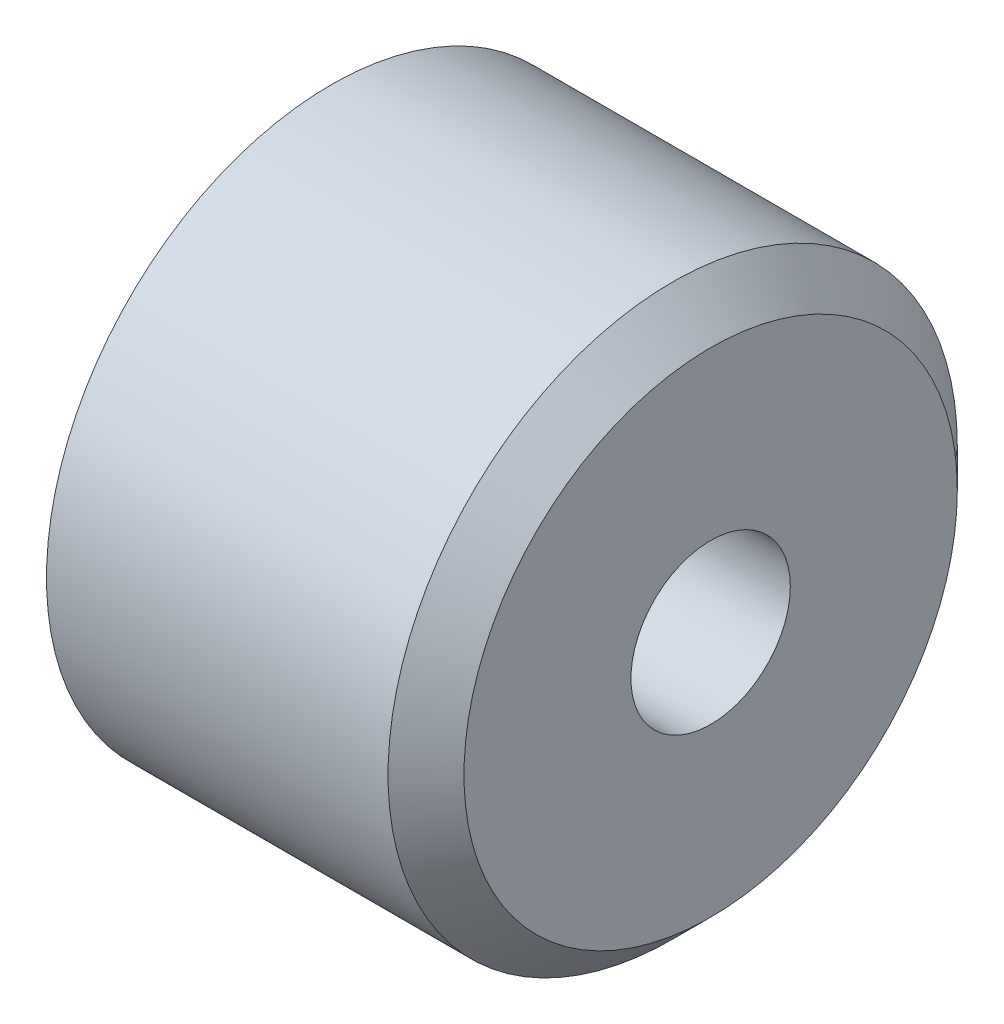
from build123d import *

# Parameters (mm, degrees)
SKETCH1_R             = 7.5
BOSS_EXTRUDE1_DEPTH   = 10
CHAMFER1_SIZE         = 1
M5_TAPPED_HOLE1_D     = 4.2
M5_TAPPED_HOLE1_DEPTH = 10
M5_TAPPED_HOLE1_TIP   = 1.2618073


with BuildPart() as part:
    # Sketch1 → Boss-Extrude1 (new body)
    with BuildSketch(Plane(origin=(2.5, 0, 0), x_dir=(0, 0, -1), z_dir=(1, 0, 0))):
        with Locations((-39.5, 200)):
            Circle(SKETCH1_R)
    extrude(amount=BOSS_EXTRUDE1_DEPTH)

    # Chamfer1
    chamfer1_edges = [part.edges().sort_by_distance(p)[0] for p in [
        (12.5, 200, 47),
    ]]
    chamfer(chamfer1_edges, length=CHAMFER1_SIZE)

    # M5 Tapped Hole1
    with Locations(Plane(origin=(12.5, 200, 39.5), x_dir=(0, 0, 1), z_dir=(1, 0, 0))):
        with Locations((0, 0)):
            Hole(M5_TAPPED_HOLE1_D / 2, depth=M5_TAPPED_HOLE1_DEPTH)
            with Locations((0, 0, -(M5_TAPPED_HOLE1_DEPTH + M5_TAPPED_HOLE1_TIP / 2))):  # 118° drill point
                Cone(0, M5_TAPPED_HOLE1_D / 2, M5_TAPPED_HOLE1_TIP, mode=Mode.SUBTRACT)


solid = part.part
